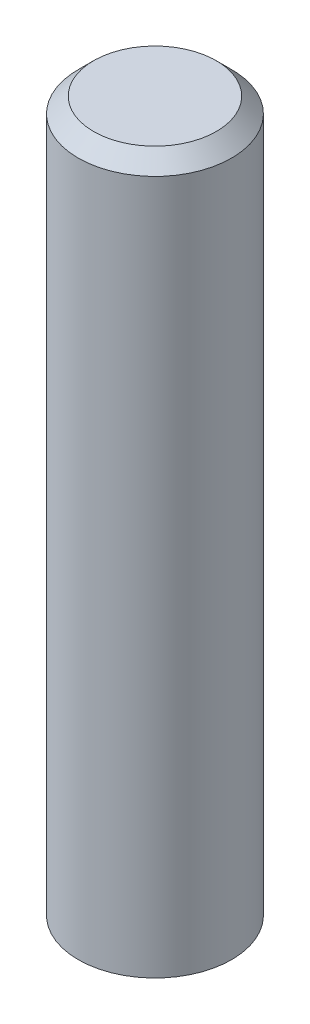
from build123d import *

# Parameters (mm, degrees)
SKETCH_1_R           = 10
BOSS_EXTRUDE_1_DEPTH = 92.5
CUT_EXTRUDE_1_DEPTH  = 95.490740287
CHAMFER_1_SIZE       = 2


with BuildPart() as part:
    # Sketch 1 → Boss-Extrude 1 (new body)
    with BuildSketch(Plane(origin=(0, 0, 0), x_dir=(1, 0, 0), z_dir=(0, 1, 0))):
        with Locations(Location((0, 0, 0), (0, 0, 270))):
            Circle(SKETCH_1_R)
    extrude(amount=BOSS_EXTRUDE_1_DEPTH)

    # Sketch 2 → Cut-Extrude 1 (cut, through all)
    with BuildSketch(Plane.XY.offset(-6.5)):
        with BuildLine():
            Line((-3, 63.5), (-3, 85.5))
            ThreePointArc((-3, 85.5), (0, 88.5), (3, 85.5))
            Line((3, 85.5), (3, 63.5))
            ThreePointArc((3, 63.5), (0, 60.5), (-3, 63.5))
        make_face()
    extrude(amount=-CUT_EXTRUDE_1_DEPTH, mode=Mode.SUBTRACT)

    # Chamfer 1
    chamfer_1_edges = [part.edges().sort_by_distance(p)[0] for p in [
        (0, 92.5, -10),
    ]]
    chamfer(chamfer_1_edges, length=CHAMFER_1_SIZE)


solid = part.part
